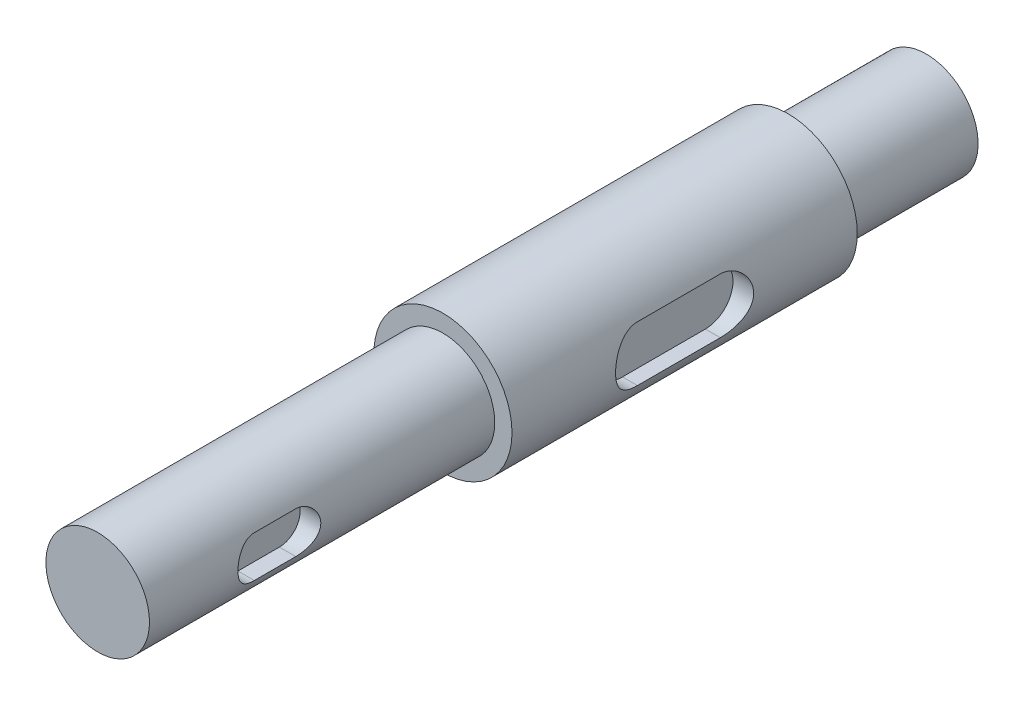
SolidWorks part; units mm, degrees
other "细节项目1"
other "标注1"
sketch "草图13" plane through (12.5, 12.5, 0) normal (0.8835, 0.4222, -0.2031) x (-0.1077, -0.2389, -0.9651)
ref_plane "前视基准面" through (0, 0, 0) normal (0, 0, 1) x (1, 0, 0)
ref_plane "上视基准面" through (0, 0, 0) normal (0, 1, 0) x (1, 0, 0)
ref_plane "右视基准面" through (0, 0, 0) normal (1, 0, 0) x (0, 0, -1)
sketch "草图1" plane through (0, 0, 0) normal (0, 0, 1) x (1, 0, 0)
  circle A0 centre (0, 0) radius 10
  dimension "D1" = 20
extrude "凸台-拉伸1" add sketch "草图1" along normal blind 60
sketch "草图3" plane through (0, 0, 60) normal (0, 0, 1) x (1, 0, 0)
  circle A0 centre (0, 0) radius 7.5
  dimension "D1" = 15
extrude "凸台-拉伸3" add sketch "草图3" along normal blind 40
sketch "草图4" plane through (0, 0, 0) normal (1, 0, 0) x (0, 0, -1)
  line L0 (-31, 0) -> (-19, 0) construction
  line L1 (13.75, 0) -> (-13.75, 0) construction
  line L2 (-31, 4) -> (-19, 4)
  line L3 (-31, -4) -> (-19, -4)
  arc A0 (-31, 4) -> (-31, -4) centre (-31, 0) ccw
  arc A1 (-19, -4) -> (-19, 4) centre (-19, 0) ccw
  point P5 (-25, 0)
  point P10 (-22.9188, 0)
  point P11 (-25, 0)
  dimension "D1" = 8
  dimension "D2" = 12
extrude "切除-拉伸1" cut sketch "草图4" against normal blind 3 from offset 10
sketch "草图10" plane through (0, 0, 60) normal (0, 0, 1) x (1, 0, 0)
  circle A0 centre (0, 0) radius 7.5
  circle A1 centre (0, 0) radius 10
extrude "切除-拉伸3" cut sketch "草图10" against normal blind 10
sketch "草图12" plane through (0, 0, 0) normal (1, 0, 0) x (0, 0, -1)
  line L0 (-84.188, 0) -> (-78.188, 0) construction
  line L1 (11, 0) -> (-11, 0) construction
  line L2 (-84.188, 3) -> (-78.188, 3)
  line L3 (-84.188, -3) -> (-78.188, -3)
  arc A0 (-84.188, 3) -> (-84.188, -3) centre (-84.188, 0) ccw
  arc A1 (-78.188, -3) -> (-78.188, 3) centre (-78.188, 0) ccw
  point P5 (-81.188, 0)
  point P10 (-124.9467, 0)
  point P11 (-161.8433, 0)
  point P12 (-142.8131, 0)
  point P13 (-81.657, 0)
  point P14 (-71.8487, 0)
  point P15 (-81.188, 0)
  dimension "D1" = 6
  dimension "D2" = 12
extrude "切除-拉伸4" cut sketch "草图12" against normal blind 3 from offset 7.5
sketch "草图14" plane through (0, 0, 0) normal (0, 0, -1) x (-1, 0, 0)
  circle A0 centre (0, 0) radius 7.5
  dimension "D1" = 15
extrude "凸台-拉伸4" add sketch "草图14" along normal blind 20
cosmetic thread "装饰螺纹线1" parameters "D2"=11.797
